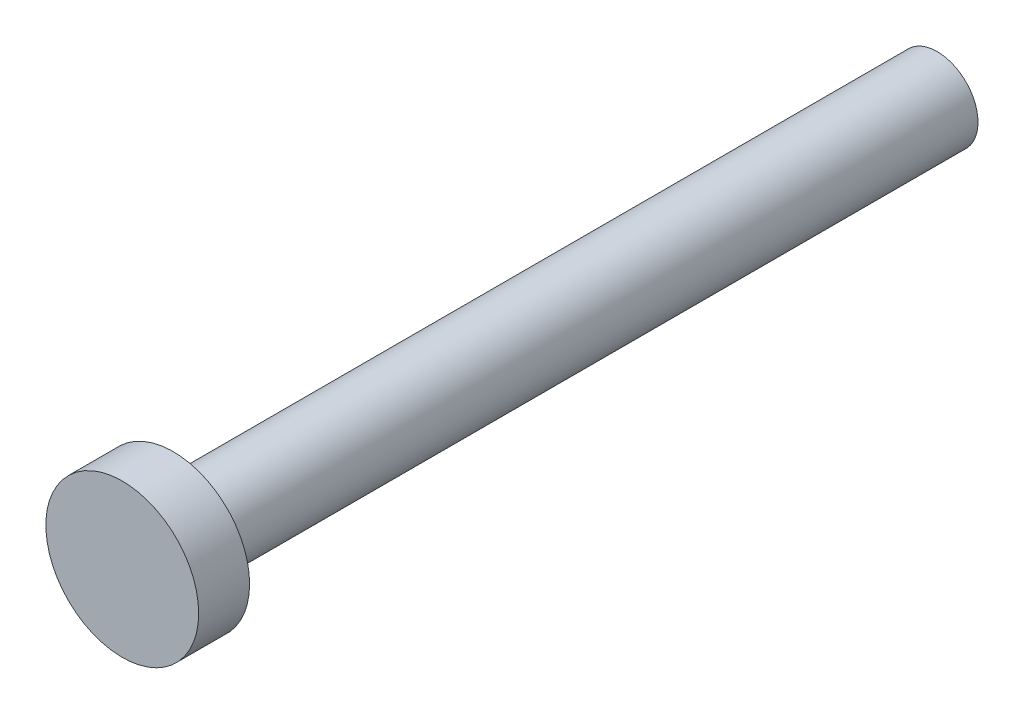
SolidWorks part; units mm, degrees
material "45"
ref_plane "Front" through (0, 0, 0) normal (0, 0, 1) x (1, 0, 0)
ref_plane "Top" through (0, 0, 0) normal (0, 1, 0) x (1, 0, 0)
ref_plane "Right" through (0, 0, 0) normal (1, 0, 0) x (0, 0, -1)
sketch "Sketch1" plane through (0, 0, 0) normal (0, 0, 1) x (1, 0, 0)
  circle A0 centre (0, 0) radius 4
  dimension "D1" = 8
extrude "Boss-Extrude1" add sketch "Sketch1" along normal blind 75
sketch "Sketch2" plane through (0, 0, 75) normal (0, 0, 1) x (1, 0, 0)
  circle A0 centre (0, 0) radius 7.5
  dimension "D1" = 15
extrude "Boss-Extrude2" add sketch "Sketch2" along normal blind 5
equation "\"零件重量\"= IIF ( \"SW-质量\" > 100 , int ( \"SW-质量\" ) , \"SW-质量\" )"
